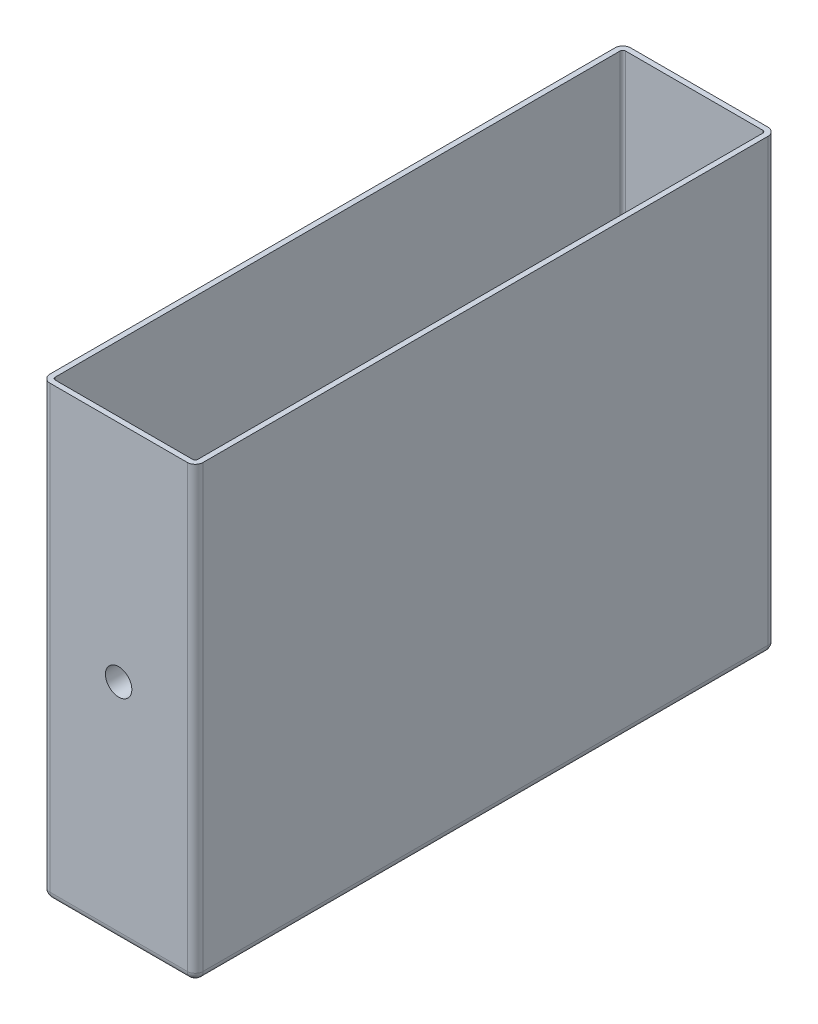
from build123d import *

# Parameters (mm, degrees)
SKETCH1_W             = 29
SKETCH1_H             = 110
BOSS_EXTRUDE1_DEPTH   = 42.5
FILLET1_R             = 1.5
SHELL1_T              = -1
SKETCH2_R             = 5
BOSS_EXTRUDE2_DEPTH   = 3
M6_TAPPED_HOLE1_D     = 5
M6_TAPPED_HOLE1_DEPTH = 4


with BuildPart() as part:
    # Sketch1 → Boss-Extrude1 (new, symmetric)
    with BuildSketch(Plane(origin=(0, 0, 0), x_dir=(1, 0, 0), z_dir=(0, 1, 0))):
        Rectangle(SKETCH1_W, SKETCH1_H)
    extrude(amount=BOSS_EXTRUDE1_DEPTH, both=True)

    # Fillet1
    fillet1_edges = [part.edges().sort_by_distance(p)[0] for p in [
        (0, -42.5, 55),
        (-14.5, -42.5, 0),
        (0, -42.5, -55),
        (14.5, -42.5, 0),
        (14.5, 0, 55),
        (-14.5, 0, 55),
        (-14.5, 0, -55),
        (14.5, 0, -55),
    ]]
    fillet(fillet1_edges, radius=FILLET1_R)

    # Shell1
    shell1_openings = [part.faces().sort_by_distance(p)[0] for p in [
        (0, 42.5, 0),
    ]]
    offset(amount=SHELL1_T, openings=shell1_openings, kind=Kind.INTERSECTION)

    # Sketch2 → Boss-Extrude2 (add)
    with BuildSketch(Plane(origin=(0, 0, 54), x_dir=(-1, 0, 0), z_dir=(0, 0, -1))):
        Circle(SKETCH2_R)
    extrude(amount=BOSS_EXTRUDE2_DEPTH)

    # M6 Tapped Hole1
    with Locations(Plane.XY.offset(55)):
        with Locations((0, 0)):
            Hole(M6_TAPPED_HOLE1_D / 2, depth=M6_TAPPED_HOLE1_DEPTH)


solid = part.part
